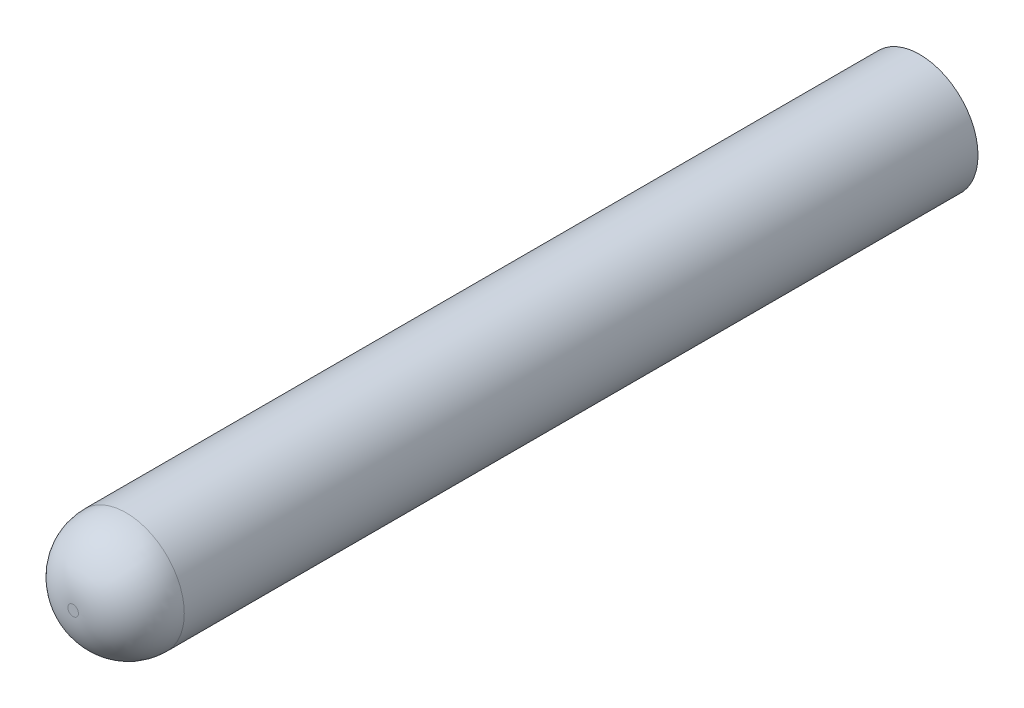
SolidWorks part; units mm, degrees
material "POM 白色"
ref_plane "Front Plane" through (0, 0, 0) normal (0, 0, 1) x (1, 0, 0)
ref_plane "Top Plane" through (0, 0, 0) normal (0, 1, 0) x (1, 0, 0)
ref_plane "Right Plane" through (0, 0, 0) normal (1, 0, 0) x (0, 0, -1)
sketch "Sketch1" plane through (0, 0, 0) normal (0, 0, 1) x (1, 0, 0)
  circle A0 centre (0, 0) radius 1.1
  dimension "D1" = 2.2
extrude "Boss-Extrude1" add sketch "Sketch1" along normal blind 16
fillet "Fillet1" radius 1 1 edges at (1.1, 0, 16)
